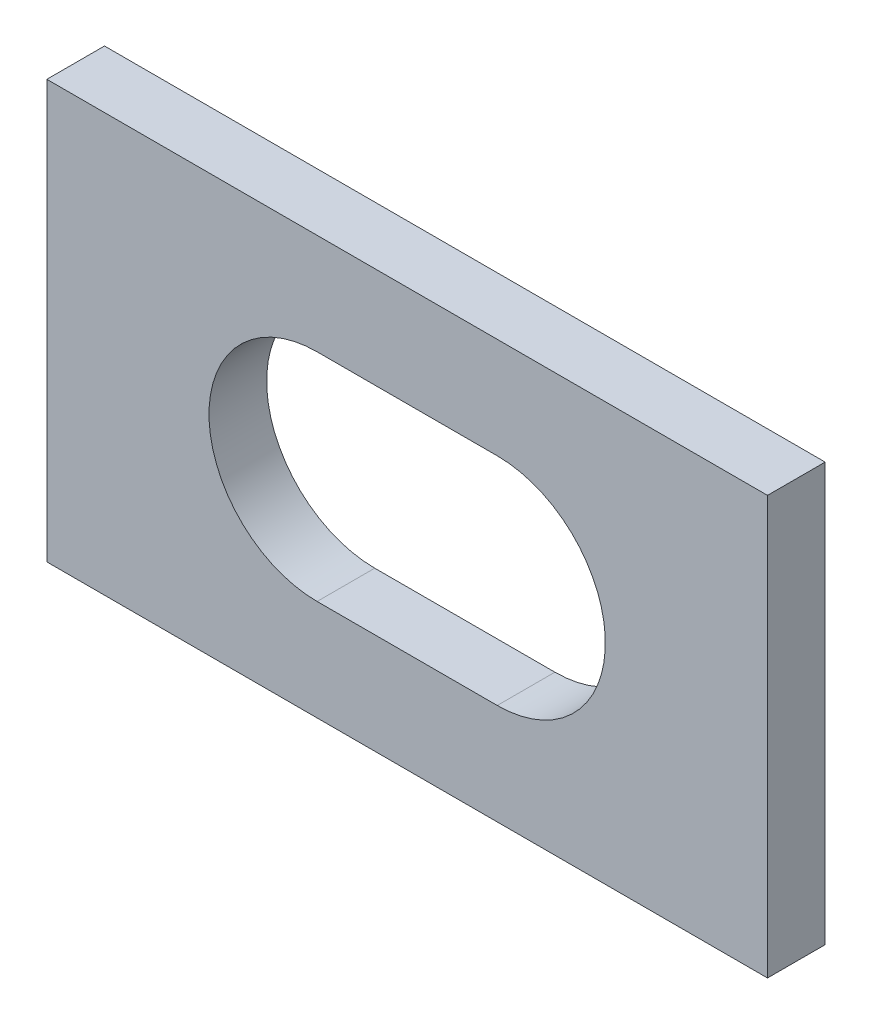
SolidWorks part; units mm, degrees
material "Q235"
ref_plane "Front Plane" through (0, 0, 0) normal (0, 0, 1) x (1, 0, 0)
ref_plane "Top Plane" through (0, 0, 0) normal (0, 1, 0) x (1, 0, 0)
ref_plane "Right Plane" through (0, 0, 0) normal (1, 0, 0) x (0, 0, -1)
sketch "Sketch1" plane through (0, 0, 0) normal (0, 0, 1) x (1, 0, 0)
  line L0 (0, 0) -> (50, 0) construction
  line L1 (0, 30) -> (50, 30)
  line L2 (0, -30) -> (50, -30)
  line L4 (-75, 58) -> (125, 58)
  line L5 (-75, 58) -> (-75, -58)
  line L6 (-75, -58) -> (125, -58)
  line L7 (125, 58) -> (125, -58)
  arc A0 (0, 30) -> (0, -30) centre (0, 0) ccw
  arc A1 (50, -30) -> (50, 30) centre (50, 0) ccw
  point P3 (25, 0)
  dimension "D4" = 30
  dimension "D1" = 200
  dimension "D2" = 116
  dimension "D3" = 50
  dimension "D5" = 58
  dimension "D6" = 100
extrude "Boss-Extrude1" add sketch "Sketch1" along normal blind 16
